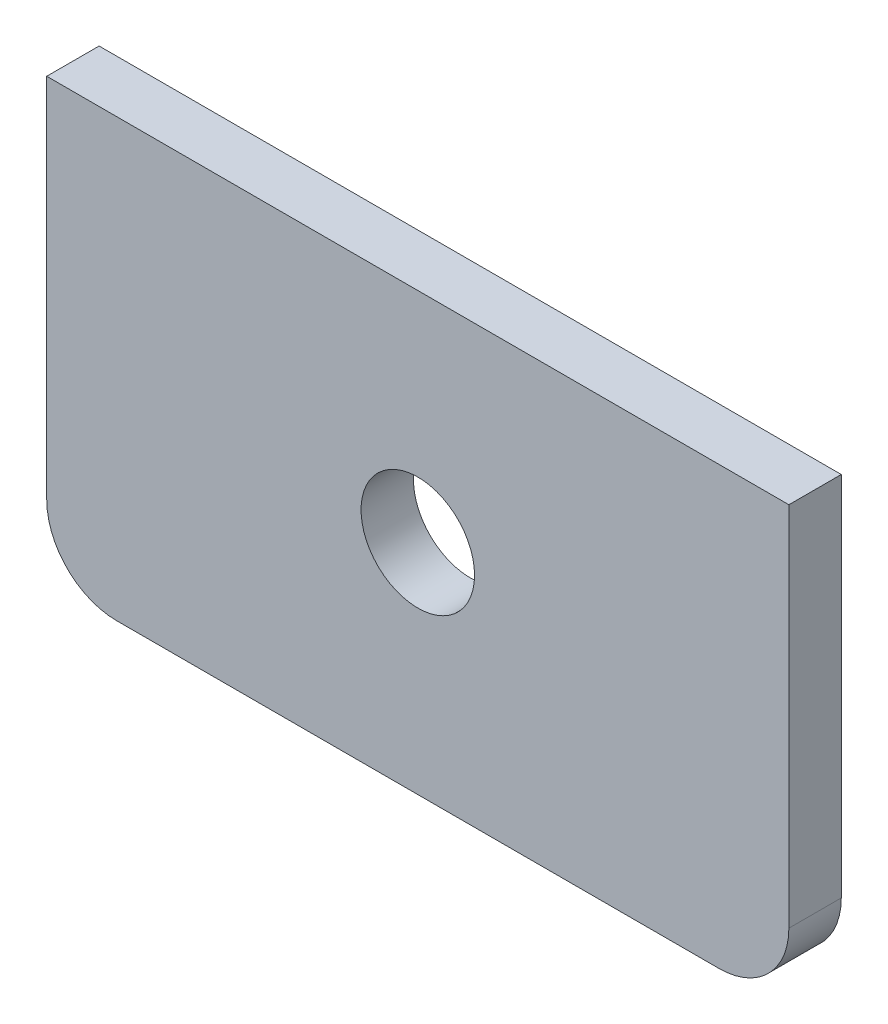
SolidWorks part; units mm, degrees
ref_plane "前视基准面" through (0, 0, 0) normal (0, 0, 1) x (1, 0, 0)
ref_plane "上视基准面" through (0, 0, 0) normal (0, 1, 0) x (1, 0, 0)
ref_plane "右视基准面" through (0, 0, 0) normal (1, 0, 0) x (0, 0, -1)
sketch "草图1" plane through (0, 0, 0) normal (0, 0, 1) x (1, 0, 0)
  line L0 (0, 0) -> (0, 10.7531) construction
  line L1 (-42.5, 25) -> (42.5, 25)
  line L2 (-42.5, 25) -> (-42.5, -17)
  line L3 (-34.5, -25) -> (34.5, -25)
  line L4 (42.5, 25) -> (42.5, -17)
  line L5 (-42.5, 25) -> (42.5, -25) construction
  line L6 (-42.5, -25) -> (42.5, 25) construction
  circle A0 centre (0, 0) radius 6.5
  arc A1 (34.5, -25) -> (42.5, -17) centre (34.5, -17) ccw
  arc A2 (-42.5, -17) -> (-34.5, -25) centre (-34.5, -17) ccw
  point P0 (0, 0)
  dimension "D3" = 13
  dimension "D4" = 25
  dimension "D5" = 8
  dimension "D1" = 85
  dimension "D2" = 50
extrude "凸台-拉伸1" add sketch "草图1" along normal blind 6
